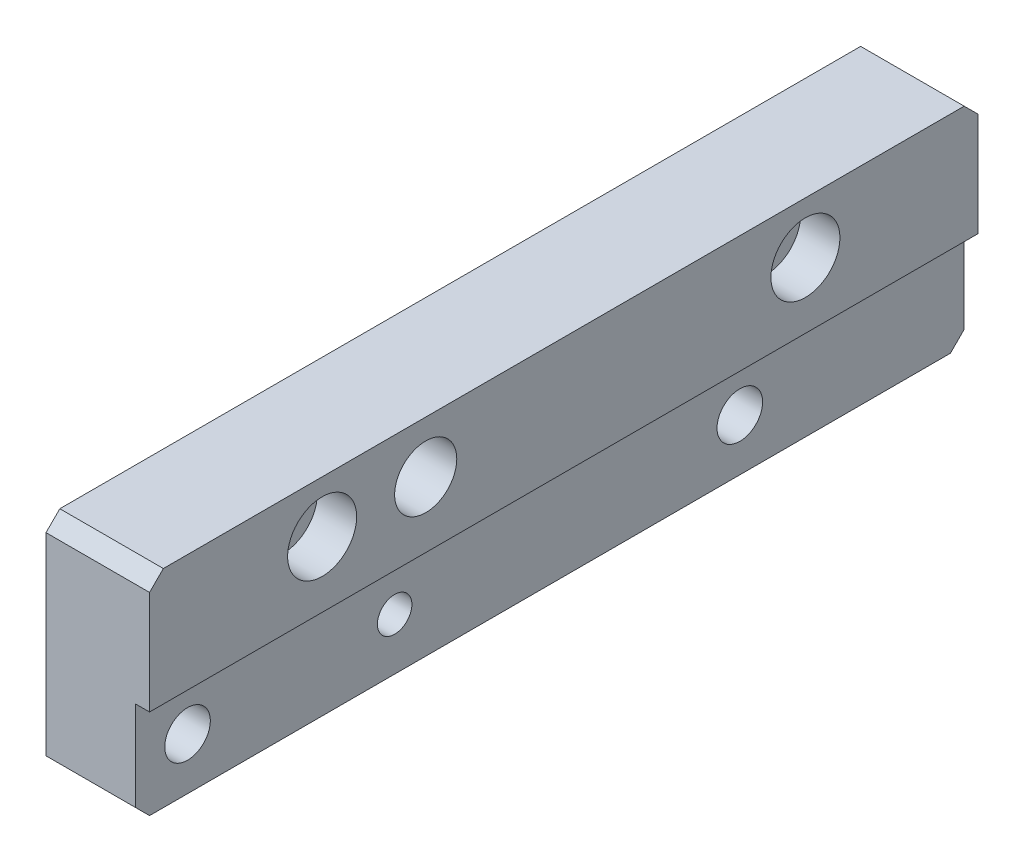
from build123d import *

# Parameters (mm, degrees)
SKETCH1_W                                            = 120
SKETCH1_H                                            = 32
BOSS_EXTRUDE1_DEPTH                                  = 15
SKETCH2_W                                            = 120
SKETCH2_H                                            = 15
CUT_EXTRUDE1_DEPTH                                   = 2
F_8_0MM_BLIND_HOLE_1_D                               = 8
F_8_0MM_BLIND_HOLE_1_DEPTH                           = 6
F_8_0MM_BLIND_HOLE_1_TIP                             = 2.403442476
M8_CLEARANCE_HOLE1_D                                 = 9
CHAMFER1_SIZE                                        = 2
CBORE_FOR_M5_HEXAGON_SOCKET_HEAD_CAP_SCR_D           = 5.5
CBORE_FOR_M5_HEXAGON_SOCKET_HEAD_CAP_SCR_CBORE_D     = 10
CBORE_FOR_M5_HEXAGON_SOCKET_HEAD_CAP_SCR_CBORE_DEPTH = 5.7
CBORE_FOR_M6_HEXAGON_SOCKET_HEAD_CAP_SCR_D           = 6.6
CBORE_FOR_M6_HEXAGON_SOCKET_HEAD_CAP_SCR_CBORE_D     = 11
CBORE_FOR_M6_HEXAGON_SOCKET_HEAD_CAP_SCR_CBORE_DEPTH = 6.8
F_5_0MM_BLIND_HOLE_1_D                               = 5


with BuildPart() as part:
    # Sketch1 → Boss-Extrude1 (new body)
    with BuildSketch(Plane(origin=(0, 0, 0), x_dir=(0, 0, -1), z_dir=(1, 0, 0))):
        Rectangle(SKETCH1_W, SKETCH1_H)
    extrude(amount=BOSS_EXTRUDE1_DEPTH)

    # Sketch2 → Cut-Extrude1 (cut)
    with BuildSketch(Plane(origin=(15, 0, 0), x_dir=(0, 0, -1), z_dir=(1, 0, 0))):
        with Locations((0, -8.5)):
            Rectangle(SKETCH2_W, SKETCH2_H)
    extrude(amount=-CUT_EXTRUDE1_DEPTH, mode=Mode.SUBTRACT)

    # Ø8.0mm blind hole 1
    with Locations(Plane.ZY):
        with Locations((35, 8.5), (-35, 8.5)):
            Hole(F_8_0MM_BLIND_HOLE_1_D / 2, depth=F_8_0MM_BLIND_HOLE_1_DEPTH)
            with Locations((0, 0, -(F_8_0MM_BLIND_HOLE_1_DEPTH + F_8_0MM_BLIND_HOLE_1_TIP / 2))):  # 118° drill point
                Cone(0, F_8_0MM_BLIND_HOLE_1_D / 2, F_8_0MM_BLIND_HOLE_1_TIP, mode=Mode.SUBTRACT)

    # M8 Clearance Hole1 (through all)
    with Locations(Plane(origin=(15, 0, 0), x_dir=(0, 0, -1), z_dir=(1, 0, 0))):
        with Locations((-20, 8.5)):
            Hole(M8_CLEARANCE_HOLE1_D / 2)

    # Chamfer1
    chamfer1_edges = [part.edges().sort_by_distance(p)[0] for p in [
        (6.5, -16, -60),
        (6.5, -16, 60),
        (7.5, 16, 60),
        (7.5, 16, -60),
    ]]
    chamfer(chamfer1_edges, length=CHAMFER1_SIZE)

    # CBORE for M5 Hexagon socket head cap screws1 (through all)
    with Locations(Plane(origin=(15, 0, 0), x_dir=(0, 0, -1), z_dir=(1, 0, 0))):
        with Locations((-35, 8.5), (35, 8.5)):
            CounterBoreHole(CBORE_FOR_M5_HEXAGON_SOCKET_HEAD_CAP_SCR_D / 2, CBORE_FOR_M5_HEXAGON_SOCKET_HEAD_CAP_SCR_CBORE_D / 2, CBORE_FOR_M5_HEXAGON_SOCKET_HEAD_CAP_SCR_CBORE_DEPTH)

    # CBORE for M6 Hexagon socket head cap screws1 (through all)
    with Locations(Plane.ZY):
        with Locations((-27.5, -8.5), (52.5, -8.5)):
            CounterBoreHole(CBORE_FOR_M6_HEXAGON_SOCKET_HEAD_CAP_SCR_D / 2, CBORE_FOR_M6_HEXAGON_SOCKET_HEAD_CAP_SCR_CBORE_D / 2, CBORE_FOR_M6_HEXAGON_SOCKET_HEAD_CAP_SCR_CBORE_DEPTH)

    # Ø5.0mm blind hole 1 (through all)
    with Locations(Plane.ZY):
        with Locations((22.5, -8.5)):
            Hole(F_5_0MM_BLIND_HOLE_1_D / 2)


solid = part.part
